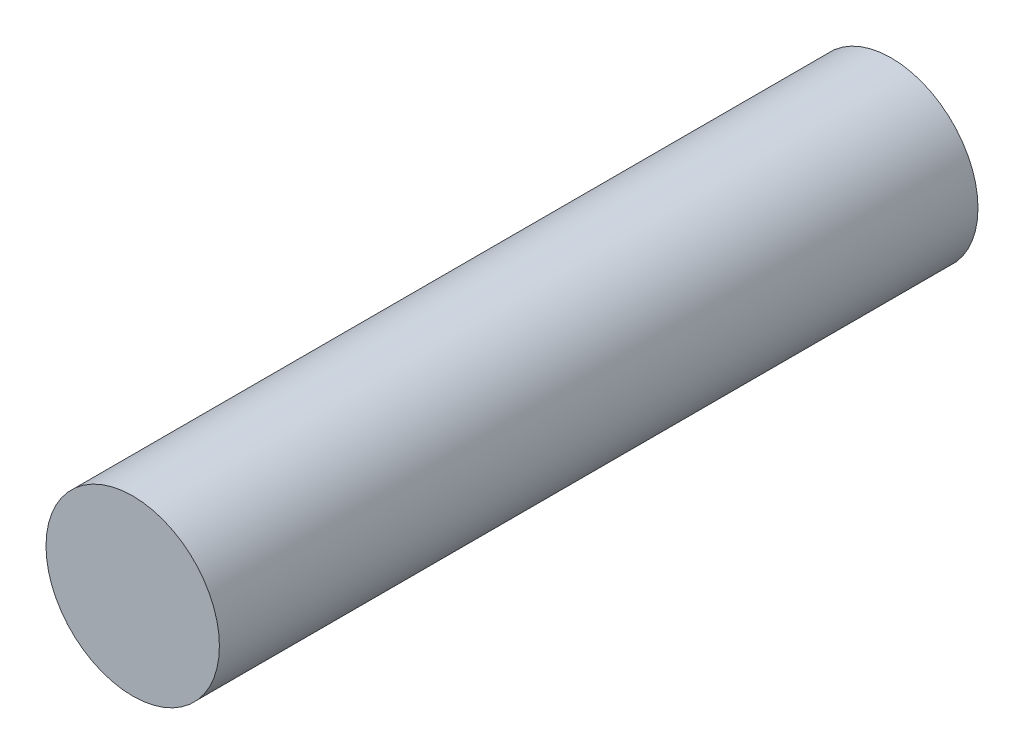
SolidWorks part; units mm, degrees
ref_plane "前视基准面" through (0, 0, 0) normal (0, 0, 1) x (1, 0, 0)
ref_plane "上视基准面" through (0, 0, 0) normal (0, 1, 0) x (1, 0, 0)
ref_plane "右视基准面" through (0, 0, 0) normal (1, 0, 0) x (0, 0, -1)
sketch "草图1" plane through (0, 0, 0) normal (0, 0, 1) x (1, 0, 0)
  circle A0 centre (0, 0) radius 4
  dimension "D1" = 8
extrude "凸台-拉伸1" add sketch "草图1" along normal blind 35
